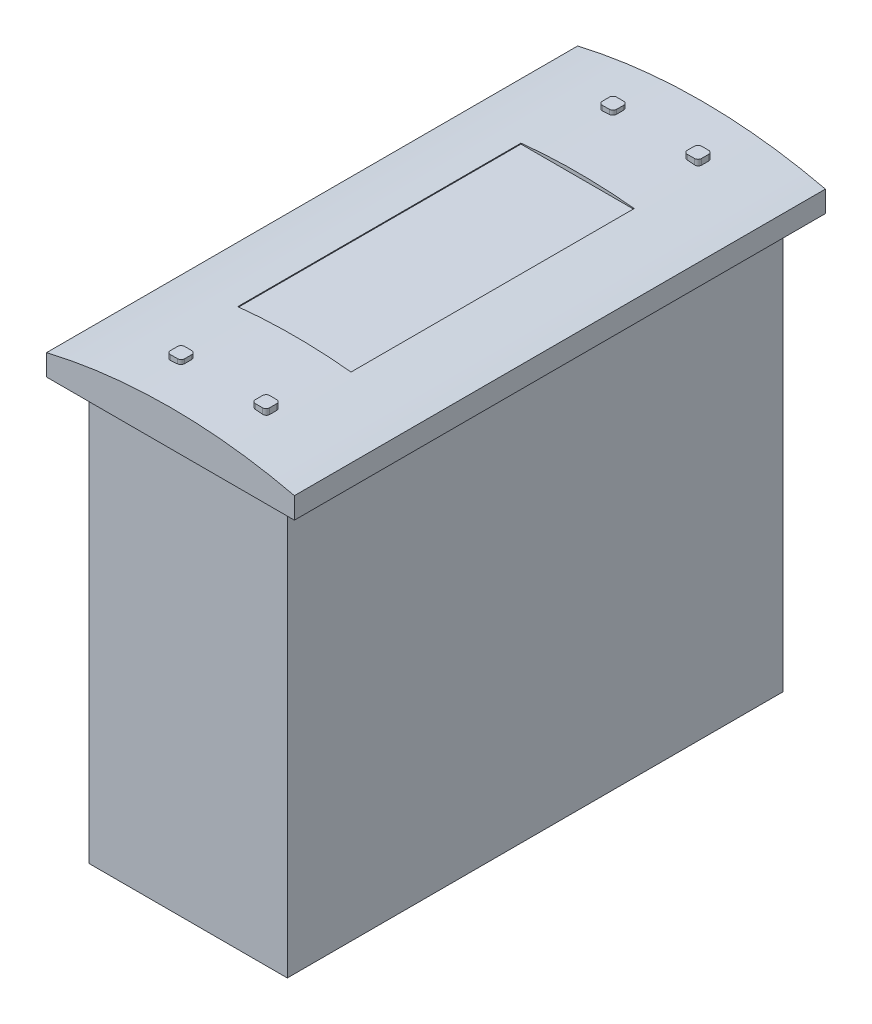
from build123d import *

# Parameters (mm, degrees)
BOSS_EXTRUDE1_DEPTH   = 75
SKETCH2_W             = 16
SKETCH2_H             = 40
CUT_EXTRUDE1_DEPTH    = 1
SKETCH4_W             = 2
SKETCH4_H             = 2
BOSS_EXTRUDE2_DEPTH   = 2.5
BOSS_EXTRUDE2_2_DEPTH = 2.5
BOSS_EXTRUDE2_3_DEPTH = 2.5
BOSS_EXTRUDE2_4_DEPTH = 2.5
FILLET1_R             = 0.5
FILLET2_R             = 0.5
FILLET3_R             = 0.5
FILLET4_R             = 0.5
SKETCH5_W             = 28
SKETCH5_H             = 70
BOSS_EXTRUDE3_DEPTH   = 59


with BuildPart() as part:
    # Sketch1 → Boss-Extrude1 (new body)
    with BuildSketch(Plane.XY):
        with BuildLine():
            Line((0, 0), (35, 0))
            Line((35, 0), (35, 3))
            ThreePointArc((35, 3), (17.5, 5.042241786), (0, 3))
            Line((0, 3), (0, 0))
        make_face()
    extrude(amount=BOSS_EXTRUDE1_DEPTH)

    # Sketch2 → Cut-Extrude1 (cut)
    with BuildSketch(Plane(origin=(0, 5.5, 0), x_dir=(1, 0, 0), z_dir=(0, 1, 0))):
        with Locations((17.5, -37.5)):
            Rectangle(SKETCH2_W, SKETCH2_H)
    extrude(amount=-CUT_EXTRUDE1_DEPTH, mode=Mode.SUBTRACT)

    # Sketch5 → Boss-Extrude3 (add)
    with BuildSketch(Plane.XZ):
        with Locations((17.5, 37.5)):
            Rectangle(SKETCH5_W, SKETCH5_H)
    extrude(amount=BOSS_EXTRUDE3_DEPTH)


with BuildPart() as body_2:
    # Sketch4 → Boss-Extrude2 (new body)
    with BuildSketch(Plane(origin=(0, 3, 0), x_dir=(-1, 0, 0), z_dir=(0, -1, 0))):
        with Locations((-12, -68)):
            Rectangle(SKETCH4_W, SKETCH4_H)
    extrude(amount=-BOSS_EXTRUDE2_DEPTH)

    # Fillet1
    fillet1_edges = [body_2.edges().sort_by_distance(p)[0] for p in [
        (11, 4.25, 69),
        (13, 4.25, 69),
        (13, 4.25, 67),
        (11, 4.25, 67),
    ]]
    fillet(fillet1_edges, radius=FILLET1_R)


with BuildPart() as body_3:
    # Sketch4 → Boss-Extrude2 2 (new body)
    with BuildSketch(Plane(origin=(0, 3, 0), x_dir=(-1, 0, 0), z_dir=(0, -1, 0))):
        with Locations((-24, -68)):
            Rectangle(SKETCH4_W, SKETCH4_H)
    extrude(amount=-BOSS_EXTRUDE2_2_DEPTH)

    # Fillet2
    fillet2_edges = [body_3.edges().sort_by_distance(p)[0] for p in [
        (23, 4.25, 69),
        (25, 4.25, 69),
        (25, 4.25, 67),
        (23, 4.25, 67),
    ]]
    fillet(fillet2_edges, radius=FILLET2_R)


with BuildPart() as body_4:
    # Sketch4 → Boss-Extrude2 3 (new body)
    with BuildSketch(Plane(origin=(0, 3, 0), x_dir=(-1, 0, 0), z_dir=(0, -1, 0))):
        with Locations((-12, -7)):
            Rectangle(SKETCH4_W, SKETCH4_H)
    extrude(amount=-BOSS_EXTRUDE2_3_DEPTH)

    # Fillet3
    fillet3_edges = [body_4.edges().sort_by_distance(p)[0] for p in [
        (11, 4.25, 8),
        (13, 4.25, 8),
        (13, 4.25, 6),
        (11, 4.25, 6),
    ]]
    fillet(fillet3_edges, radius=FILLET3_R)


with BuildPart() as body_5:
    # Sketch4 → Boss-Extrude2 4 (new body)
    with BuildSketch(Plane(origin=(0, 3, 0), x_dir=(-1, 0, 0), z_dir=(0, -1, 0))):
        with Locations((-24, -7)):
            Rectangle(SKETCH4_W, SKETCH4_H)
    extrude(amount=-BOSS_EXTRUDE2_4_DEPTH)

    # Fillet4
    fillet4_edges = [body_5.edges().sort_by_distance(p)[0] for p in [
        (23, 4.25, 8),
        (25, 4.25, 8),
        (25, 4.25, 6),
        (23, 4.25, 6),
    ]]
    fillet(fillet4_edges, radius=FILLET4_R)


solid = Compound([part.part, body_2.part, body_3.part, body_4.part, body_5.part])
